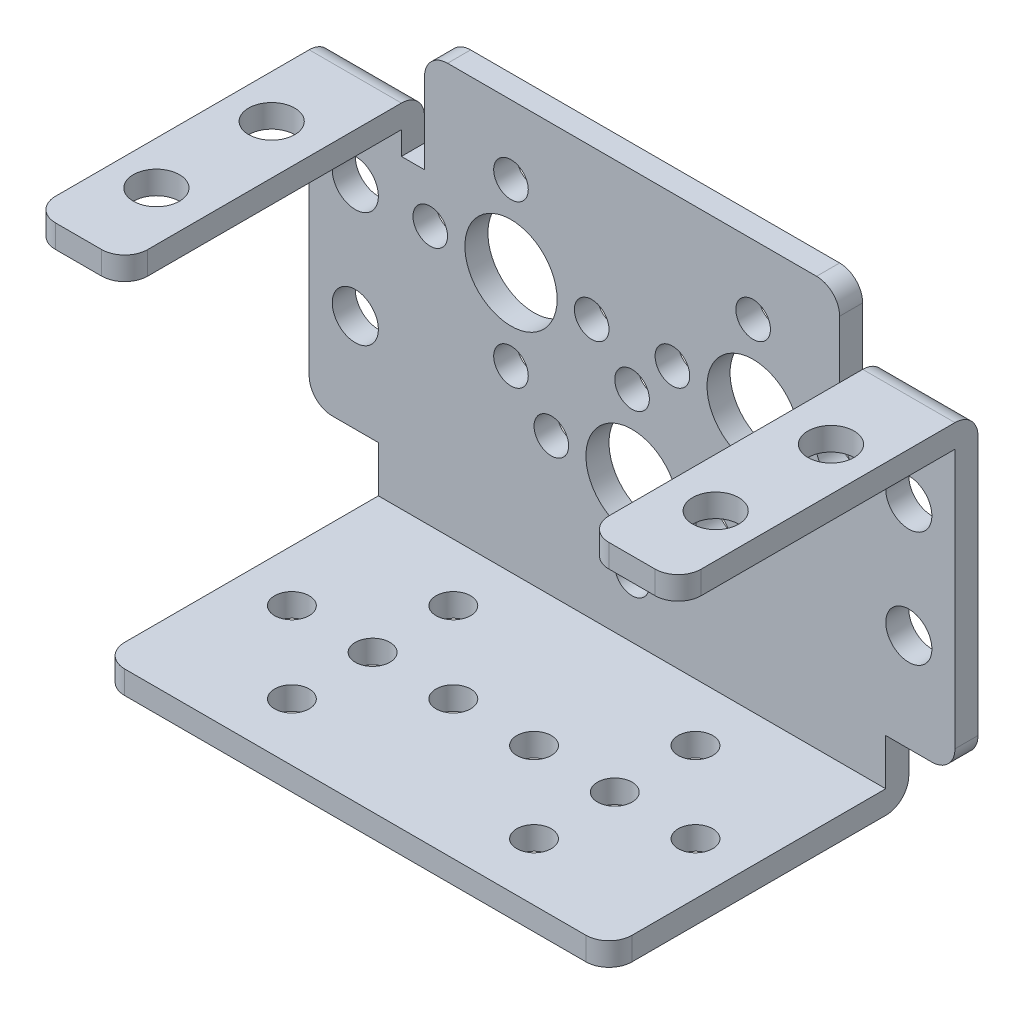
from build123d import *

# Parameters (mm, degrees)
SKETCH3_W           = 56
SKETCH3_H           = 37.49
BOSS_EXTRUDE1_DEPTH = 2
SKETCH4_W           = 56
SKETCH4_H           = 2
BOSS_EXTRUDE2_DEPTH = 24
SKETCH5_W           = 8
SKETCH5_H           = 2
BOSS_EXTRUDE3_DEPTH = 24
LINPATTERN1_COUNT   = 2
LINPATTERN1_PITCH   = 48
SKETCH6_W           = 6
SKETCH6_H           = 6
CUT_EXTRUDE1_DEPTH  = 42.368768715
LINPATTERN2_COUNT   = 2
LINPATTERN2_PITCH   = 50
CUT_EXTRUDE2_DEPTH  = 23.5
CUT_EXTRUDE3_DEPTH  = 23.5
SKETCH9_R           = 2
SKETCH9_R_2         = 4
SKETCH9_R_3         = 1.5
CUT_EXTRUDE4_DEPTH  = 23.5
SKETCH11_R          = 1.5
CUT_EXTRUDE5_DEPTH  = 53.149209965
FILLET1_R           = 2
SKETCH12_R          = 2
CUT_EXTRUDE6_DEPTH  = 23.5


with BuildPart() as part:
    # Sketch3 → Boss-Extrude1 (new body)
    with BuildSketch(Plane.XY):
        Rectangle(SKETCH3_W, SKETCH3_H)
    extrude(amount=BOSS_EXTRUDE1_DEPTH)

    # Sketch4 → Boss-Extrude2 (add)
    with BuildSketch(Plane.XY.offset(2)):
        with Locations((0, -17.745)):
            Rectangle(SKETCH4_W, SKETCH4_H)
    extrude(amount=BOSS_EXTRUDE2_DEPTH)

    # Sketch5 → Boss-Extrude3 (add)
    with BuildSketch(Plane.XY.offset(2)):
        with Locations((-24, 12.755)):
            Rectangle(SKETCH5_W, SKETCH5_H)
    boss_extrude3 = extrude(amount=BOSS_EXTRUDE3_DEPTH)

    # LinPattern1: Boss-Extrude3 ×2
    with Locations(*[(i * LINPATTERN1_PITCH, 0, 0) for i in range(1, LINPATTERN1_COUNT)]):
        add(boss_extrude3)

    # Sketch6 → Cut-Extrude1 (cut, symmetric)
    with BuildSketch(Plane.XY.offset(2)):
        with Locations((-25, -15.745)):
            Rectangle(SKETCH6_W, SKETCH6_H)
    cut_extrude1 = extrude(amount=CUT_EXTRUDE1_DEPTH, both=True, mode=Mode.SUBTRACT)

    # LinPattern2: Cut-Extrude1 ×2
    with Locations(*[(i * LINPATTERN2_PITCH, 0, 0) for i in range(1, LINPATTERN2_COUNT)]):
        add(cut_extrude1, mode=Mode.SUBTRACT)

    # Sketch7 → Cut-Extrude2 (cut)
    with BuildSketch(Plane.XY.offset(2)):
        Polygon((-28, 18.745), (-28, 13.755), (-20, 13.755), (-20, 11.755), (-20, 9.745), (-18, 9.745), (-18, 18.745), align=None)
    extrude(amount=-CUT_EXTRUDE2_DEPTH, mode=Mode.SUBTRACT)

    # Sketch8 → Cut-Extrude3 (cut)
    with BuildSketch(Plane.XY.offset(2)):
        Polygon((28, 13.755), (28, 18.745), (18, 18.745), (18, 9.745), (20, 9.745), (20, 13.755), align=None)
    extrude(amount=-CUT_EXTRUDE3_DEPTH, mode=Mode.SUBTRACT)

    # Sketch9 → Cut-Extrude4 (cut)
    with BuildSketch(Plane.XY.offset(2)):
        with Locations((-24, 5.755)):
            Circle(SKETCH9_R)
        with Locations((-24, -4.245)):
            Circle(SKETCH9_R)
        with Locations((-10.5, 5.755)):
            Circle(SKETCH9_R_2)
        with Locations((0, -4.745)):
            Circle(SKETCH9_R_2)
        with Locations((0, 2.255)):
            Circle(SKETCH9_R_3)
        with Locations((0, -11.745)):
            Circle(SKETCH9_R_3)
        with Locations((-10.5, -1.245)):
            Circle(SKETCH9_R_3)
        with Locations((-10.5, 12.755)):
            Circle(SKETCH9_R_3)
        with Locations((-17.5, 5.755)):
            Circle(SKETCH9_R_3)
        with Locations((-3.5, 5.755)):
            Circle(SKETCH9_R_3)
        with Locations((-7, -4.745)):
            Circle(SKETCH9_R_3)
        with Locations((7, -4.745)):
            Circle(SKETCH9_R_3)
        with Locations((10.5, 12.755)):
            Circle(SKETCH9_R_3)
        with Locations((3.5, 5.755)):
            Circle(SKETCH9_R_3)
        with Locations((10.5, -1.245)):
            Circle(SKETCH9_R_3)
        with Locations((10.5, 5.755)):
            Circle(SKETCH9_R_2)
        with Locations((17.5, 5.755)):
            Circle(SKETCH9_R_3)
        with Locations((24, -4.245)):
            Circle(SKETCH9_R)
        with Locations((24, 5.755)):
            Circle(SKETCH9_R)
    extrude(amount=-CUT_EXTRUDE4_DEPTH, mode=Mode.SUBTRACT)

    # Sketch11 → Cut-Extrude5 (cut, through all)
    with BuildSketch(Plane(origin=(0, -16.745, 0), x_dir=(1, 0, 0), z_dir=(0, 1, 0))):
        with Locations(Location((-10.5, -14, 0), (0, 0, 270))):
            Circle(SKETCH11_R)
        with Locations(Location((-17.5, -14, 0), (0, 0, 270))):
            Circle(SKETCH11_R)
        with Locations(Location((-10.5, -21, 0), (0, 0, 270))):
            Circle(SKETCH11_R)
        with Locations(Location((-3.5, -14, 0), (0, 0, 270))):
            Circle(SKETCH11_R)
        with Locations(Location((-10.5, -7, 0), (0, 0, 270))):
            Circle(SKETCH11_R)
        with Locations(Location((10.5, -21, 0), (0, 0, 90))):
            Circle(SKETCH11_R)
        with Locations(Location((3.5, -14, 0), (0, 0, 90))):
            Circle(SKETCH11_R)
        with Locations(Location((10.5, -7, 0), (0, 0, 90))):
            Circle(SKETCH11_R)
        with Locations(Location((10.5, -14, 0), (0, 0, 90))):
            Circle(SKETCH11_R)
        with Locations(Location((17.5, -14, 0), (0, 0, 90))):
            Circle(SKETCH11_R)
    extrude(amount=-CUT_EXTRUDE5_DEPTH, mode=Mode.SUBTRACT)

    # Fillet1
    fillet1_edges = [part.edges().sort_by_distance(p)[0] for p in [
        (-24, 13.755, 0),
        (-18, 18.745, 1),
        (24, 13.755, 0),
        (18, 18.745, 1),
        (-28, 12.755, 26),
        (-20, 12.755, 26),
        (20, 12.755, 26),
        (28, 12.755, 26),
        (-22, -17.745, 26),
        (0, -18.745, 0),
        (-28, -12.745, 1),
        (22, -17.745, 26),
        (28, -12.745, 1),
    ]]
    fillet(fillet1_edges, radius=FILLET1_R)

    # Sketch12 → Cut-Extrude6 (cut)
    with BuildSketch(Plane(origin=(0, 13.755, 0), x_dir=(1, 0, 0), z_dir=(0, 1, 0))):
        with Locations(Location((-24.25, -19, 0), (0, 0, 270))):
            Circle(SKETCH12_R)
        with Locations(Location((-24.25, -9, 0), (0, 0, 270))):
            Circle(SKETCH12_R)
    cut_extrude6 = extrude(amount=-CUT_EXTRUDE6_DEPTH, mode=Mode.SUBTRACT)

    # Mirror2: Cut-Extrude6 across plane
    add(cut_extrude6.mirror(Plane(origin=(0, 0, 0), x_dir=(0, 0, 1), z_dir=(1, 0, 0))), mode=Mode.SUBTRACT)


solid = part.part
